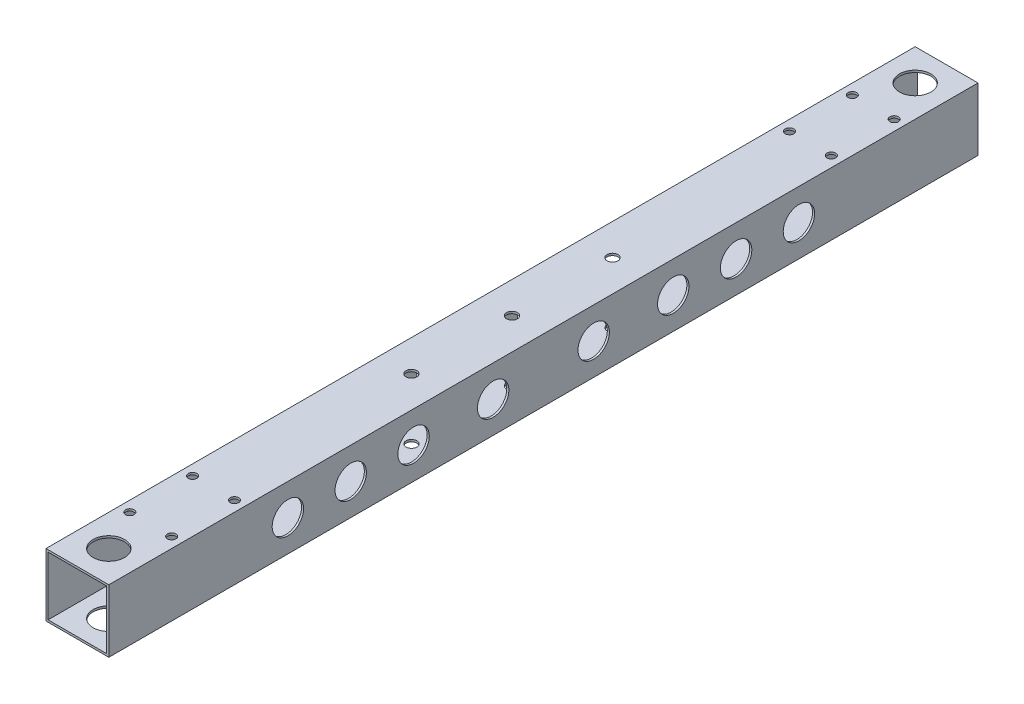
from build123d import *

# Parameters (mm, degrees)
SKETCH_1_W          = 30
SKETCH_1_H          = 30
EXTRUDE_1_DEPTH     = 415
SHELL_1_T           = -1
SKETCH_2_R          = 2.6
SKETCH_2_R_2        = 2.05
CUT_EXTRUDE_1_DEPTH = 417.353215431
SKETCH_3_R          = 7.5
CUT_EXTRUDE_2_DEPTH = 417.353215431
SKETCH_4_R          = 7.5
CUT_EXTRUDE_3_DEPTH = 417.353215431


with BuildPart() as part:
    # 草图1 → 凸台-拉伸1 (new body)
    with BuildSketch(Plane.XY):
        Rectangle(SKETCH_1_W, SKETCH_1_H)
    extrude(amount=EXTRUDE_1_DEPTH)

    # 抽壳1
    shell_1_openings = [part.faces().sort_by_distance(p)[0] for p in [
        (0, 0, 415),
        (0, 0, 0),
    ]]
    offset(amount=SHELL_1_T, openings=shell_1_openings, kind=Kind.INTERSECTION)

    # 草图2 → 切除-拉伸1 (cut, through all)
    with BuildSketch(Plane(origin=(0, 15, 0), x_dir=(1, 0, 0), z_dir=(0, 1, 0))):
        with Locations(Location((0, -159.5, 0), (0, 0, 270))):
            Circle(SKETCH_2_R)
        with Locations(Location((0, -255.5, 0), (0, 0, 270))):
            Circle(SKETCH_2_R)
        with Locations(Location((0, -207.5, 0), (0, 0, 270))):
            Circle(SKETCH_2_R)
        with Locations(Location((-10, -35, 0), (0, 0, 270))):
            Circle(SKETCH_2_R_2)
        with Locations(Location((-10, -380, 0), (0, 0, 90))):
            Circle(SKETCH_2_R_2)
        with Locations(Location((-10, -65, 0), (0, 0, 270))):
            Circle(SKETCH_2_R_2)
        with Locations(Location((-10, -350, 0), (0, 0, 90))):
            Circle(SKETCH_2_R_2)
        with Locations(Location((10, -65, 0), (0, 0, 270))):
            Circle(SKETCH_2_R_2)
        with Locations(Location((10, -350, 0), (0, 0, 90))):
            Circle(SKETCH_2_R_2)
        with Locations(Location((10, -35, 0), (0, 0, 270))):
            Circle(SKETCH_2_R_2)
        with Locations(Location((10, -380, 0), (0, 0, 90))):
            Circle(SKETCH_2_R_2)
    extrude(amount=-CUT_EXTRUDE_1_DEPTH, mode=Mode.SUBTRACT)

    # 草图3 → 切除-拉伸2 (cut, through all)
    with BuildSketch(Plane.ZY.offset(15)):
        with Locations((85.5, 0)):
            Circle(SKETCH_3_R)
        with Locations((115.5, 0)):
            Circle(SKETCH_3_R)
        with Locations((145.5, 0)):
            Circle(SKETCH_3_R)
        with Locations((269.5, 0)):
            Circle(SKETCH_3_R)
        with Locations((299.5, 0)):
            Circle(SKETCH_3_R)
        with Locations((329.5, 0)):
            Circle(SKETCH_3_R)
        with Locations((183.5, 0)):
            Circle(SKETCH_3_R)
        with Locations((231.5, 0)):
            Circle(SKETCH_3_R)
    extrude(amount=-CUT_EXTRUDE_2_DEPTH, mode=Mode.SUBTRACT)

    # 草图4 → 切除-拉伸3 (cut, through all)
    with BuildSketch(Plane(origin=(0, 15, 0), x_dir=(1, 0, 0), z_dir=(0, 1, 0))):
        with Locations(Location((0, -15, 0), (0, 0, 270))):
            Circle(SKETCH_4_R)
        with Locations(Location((0, -400, 0), (0, 0, 90))):
            Circle(SKETCH_4_R)
    extrude(amount=-CUT_EXTRUDE_3_DEPTH, mode=Mode.SUBTRACT)


solid = part.part
